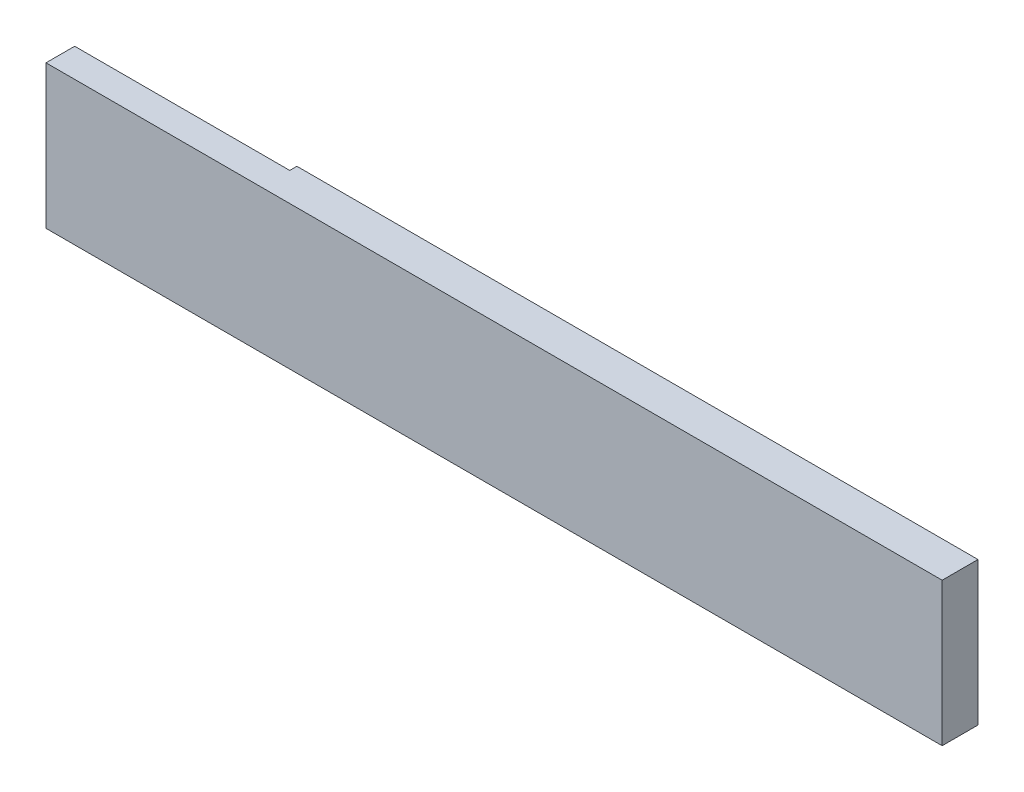
from build123d import *

# Parameters (mm, degrees)
SKETCH_1_W          = 250
SKETCH_1_H          = 40
EXTRUDE_1_DEPTH     = 5
SKETCH_2_W          = 60
SKETCH_2_H          = 40
CUT_EXTRUDE_1_DEPTH = 2


with BuildPart() as part:
    # 草图1 → 凸台-拉伸1 (new, symmetric)
    with BuildSketch(Plane.XY):
        Rectangle(SKETCH_1_W, SKETCH_1_H)
    extrude(amount=EXTRUDE_1_DEPTH, both=True)

    # 草图2 → 切除-拉伸1 (cut)
    with BuildSketch(Plane(origin=(0, 0, -5), x_dir=(-1, 0, 0), z_dir=(0, 0, -1))):
        with Locations((95, 0)):
            Rectangle(SKETCH_2_W, SKETCH_2_H)
    extrude(amount=-CUT_EXTRUDE_1_DEPTH, mode=Mode.SUBTRACT)


solid = part.part
